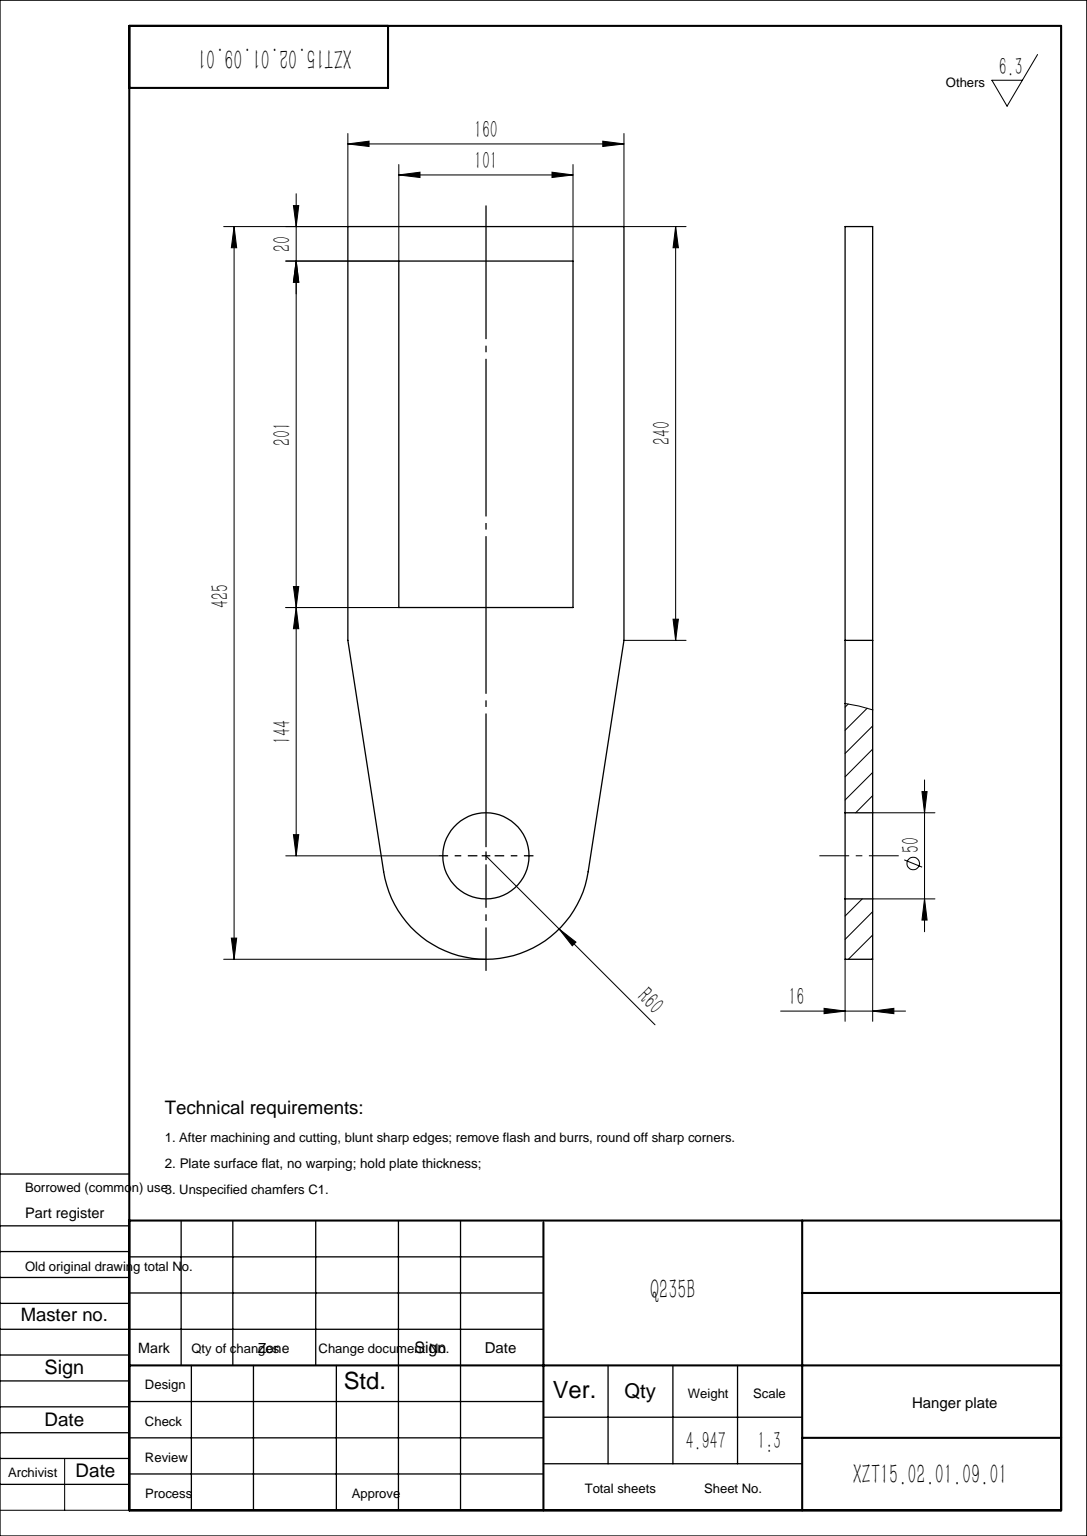
SolidWorks part; units mm, degrees
material "Q235B"
ref_plane "Front Plane" through (0, 0, 0) normal (0, 0, 1) x (1, 0, 0)
ref_plane "Top Plane" through (0, 0, 0) normal (0, 1, 0) x (1, 0, 0)
ref_plane "Right Plane" through (0, 0, 0) normal (1, 0, 0) x (0, 0, -1)
sketch "Sketch1" plane through (0, 0, 0) normal (0, 0, 1) x (1, 0, 0)
  line L0 (0, 0) -> (0, 365) construction
  line L1 (80, 365) -> (-80, 365)
  line L2 (-80, 365) -> (-80, 125)
  line L3 (-80, 125) -> (-59.2981, -9.1508)
  line L4 (80, 125) -> (59.2981, -9.1508)
  line L5 (80, 365) -> (80, 125)
  line L7 (50.5, 144) -> (-50.5, 144)
  line L8 (50.5, 144) -> (50.5, 345)
  line L9 (50.5, 345) -> (-50.5, 345)
  line L10 (-50.5, 144) -> (-50.5, 345)
  line L11 (50.5, 144) -> (-50.5, 345) construction
  line L12 (50.5, 345) -> (-50.5, 144) construction
  arc A0 (-59.2981, -9.1508) -> (0, -60) centre (0, 0) ccw
  arc A1 (59.2981, -9.1508) -> (0, -60) centre (0, 0) cw
  circle A2 centre (0, 0) radius 25
  point P14 (0, 244.5)
  dimension "D1" = 425
  dimension "D2" = 60
  dimension "D8" = 50
  dimension "D3" = 240
  dimension "D4" = 160
  dimension "D5" = 201
  dimension "D6" = 20
  dimension "D7" = 101
extrude "Boss-Extrude1" add sketch "Sketch1" along normal mid plane 16
